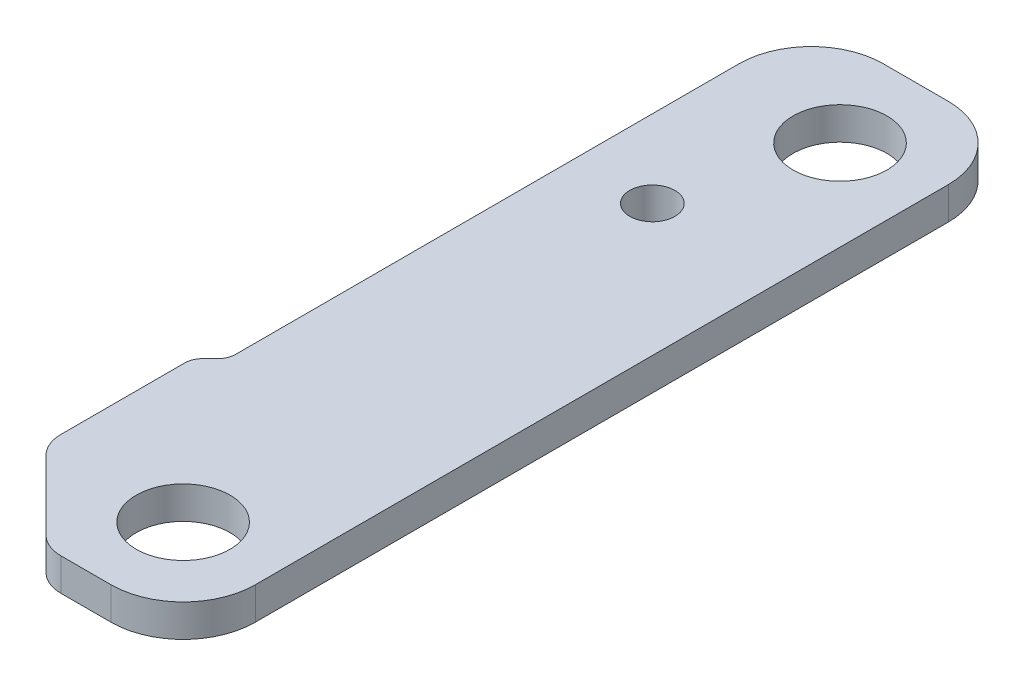
from build123d import *

# Parameters (mm, degrees)
SKETCH1_R           = 13
SKETCH1_R_2         = 6.25
BOSS_EXTRUDE1_DEPTH = 9


with BuildPart() as part:
    # Sketch1 → Boss-Extrude1 (new body)
    with BuildSketch(Plane(origin=(0, 0, 0), x_dir=(1, 0, 0), z_dir=(0, 1, 0))):
        with BuildLine():
            Line((2.928932188, 22.071067812), (22.071067812, 2.928932188))
            ThreePointArc((22.071067812, 2.928932188), (25.3153013, 0.761204675), (29.142135624, 0))
            Line((29.142135624, 0), (43, 0))
            ThreePointArc((43, 0), (57.142135624, 5.857864376), (63, 20))
            Line((63, 20), (63, 212))
            ThreePointArc((63, 212), (57.142135624, 226.142135624), (43, 232))
            Line((43, 232), (25, 232))
            ThreePointArc((25, 232), (10.857864376, 226.142135624), (5, 212))
            Line((5, 212), (5, 72.571067812))
            ThreePointArc((5, 72.571067812), (4.619397663, 70.65765065), (3.535533906, 69.035533906))
            Line((3.535533906, 69.035533906), (1.464466094, 66.964466094))
            ThreePointArc((1.464466094, 66.964466094), (0.380602337, 65.34234935), (0, 63.428932188))
            Line((0, 63.428932188), (0, 29.142135624))
            ThreePointArc((0, 29.142135624), (0.761204675, 25.3153013), (2.928932188, 22.071067812))
        make_face()
        with Locations(Location((38, 25, 0), (0, 0, 270))):
            Circle(SKETCH1_R, mode=Mode.SUBTRACT)
        with Locations(Location((38, 207, 0), (0, 0, 270))):
            Circle(SKETCH1_R, mode=Mode.SUBTRACT)
        with Locations(Location((26.5, 166.5, 0), (0, 0, 270))):
            Circle(SKETCH1_R_2, mode=Mode.SUBTRACT)
    extrude(amount=BOSS_EXTRUDE1_DEPTH)


solid = part.part
